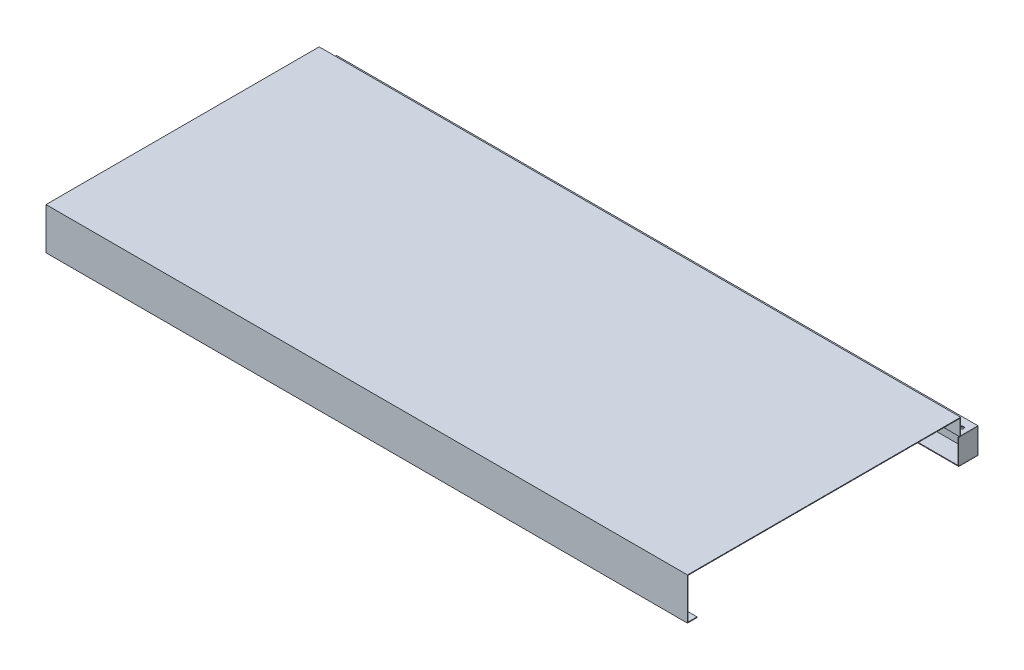
from build123d import *

# Parameters (mm, degrees)
EXTRUDE_THIN1_DEPTH = 998
SKETCH4_W           = 29
SKETCH4_H           = 38
EXTRUDE2_DEPTH      = 1
SKETCH5_W           = 29
SKETCH5_H           = 38
EXTRUDE3_DEPTH      = 1
SKETCH6_R           = 2.75
CUT_EXTRUDE1_DEPTH  = 10


with BuildPart() as part:
    # Sketch1 → Extrude-Thin1 (new body)
    with BuildSketch(Plane(origin=(0, 0, 0), x_dir=(0, 0, -1), z_dir=(1, 0, 0))):
        Polygon((-35, -65), (-50, -65), (-50, 0), (0, 0), (375, 0), (375, -25), (402, -25), (402, -65), (372, -65), (372, -64), (401, -64), (401, -26), (374, -26), (374, -1), (0, -1), (-49, -1), (-49, -64), (-35, -64), align=None)
    extrude(amount=EXTRUDE_THIN1_DEPTH)

    # Sketch6 → Cut-Extrude1 (cut)
    with BuildSketch(Plane(origin=(0, -25, 0), x_dir=(1, 0, 0), z_dir=(0, 1, 0))):
        with Locations(Location((13, 389, 0), (0, 0, 270))):
            Circle(SKETCH6_R)
        with Locations(Location((988, 387, 0), (0, 0, 270))):
            Circle(SKETCH6_R)
    extrude(amount=-CUT_EXTRUDE1_DEPTH, mode=Mode.SUBTRACT)


with BuildPart() as body_2:
    # Sketch4 → Extrude2 (new body)
    with BuildSketch(Plane.ZY):
        with Locations((-386.5, -45)):
            Rectangle(SKETCH4_W, SKETCH4_H)
    extrude(amount=-EXTRUDE2_DEPTH)


with BuildPart() as body_3:
    # Sketch5 → Extrude3 (new body)
    with BuildSketch(Plane(origin=(998, 0, 0), x_dir=(0, 0, -1), z_dir=(1, 0, 0))):
        with Locations((386.5, -45)):
            Rectangle(SKETCH5_W, SKETCH5_H)
    extrude(amount=-EXTRUDE3_DEPTH)


solid = Compound([part.part, body_2.part, body_3.part])
